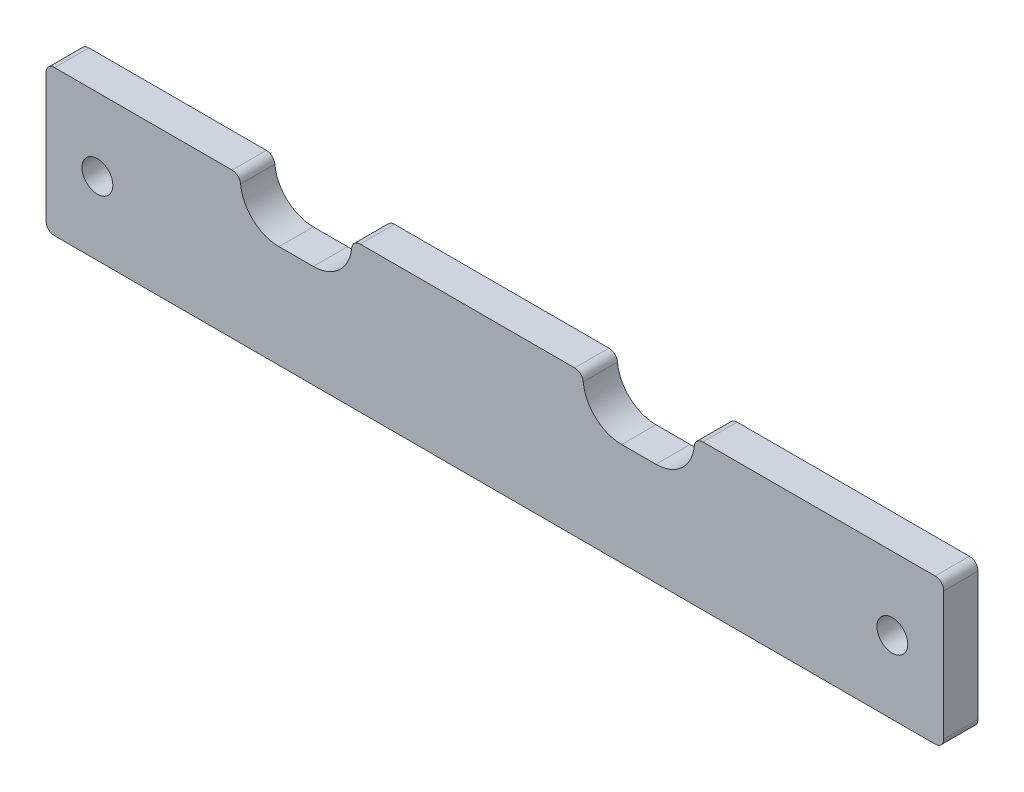
SolidWorks part; units mm, degrees
material "Q235B"
ref_plane "Front Plane" through (0, 0, 0) normal (0, 0, 1) x (1, 0, 0)
ref_plane "Top Plane" through (0, 0, 0) normal (0, 1, 0) x (1, 0, 0)
ref_plane "Right Plane" through (0, 0, 0) normal (1, 0, 0) x (0, 0, -1)
sketch "Sketch1" plane through (0, 0, 0) normal (0, 0, 1) x (1, 0, 0)
  line L0 (-26685.0454, 9467.9632) -> (-26685.0454, 9542.9632)
  line L1 (-26161.0454, 9467.9632) -> (-26161.0454, 9542.9632)
  line L2 (-26166.0454, 9462.9632) -> (-26680.0454, 9462.9632)
  line L3 (-26549.0454, 9522.9632) -> (-26529.0454, 9522.9632)
  line L4 (-26349.0454, 9522.9632) -> (-26329.0454, 9522.9632)
  line L5 (-26680.0454, 9547.9632) -> (-26576.4315, 9547.9632)
  line L6 (-26501.6593, 9547.9632) -> (-26376.4315, 9547.9632)
  line L7 (-26301.6593, 9547.9632) -> (-26289.0454, 9547.9632)
  line L8 (-26289.0454, 9547.9632) -> (-26166.0454, 9547.9632)
  circle A0 centre (-26655.0454, 9505.4632) radius 9
  circle A1 centre (-26191.0454, 9505.4632) radius 9
  arc A2 (-26571.4522, 9543.4178) -> (-26549.0454, 9522.9632) centre (-26549.0454, 9545.4632) ccw
  arc A3 (-26529.0454, 9522.9632) -> (-26506.6386, 9543.4178) centre (-26529.0454, 9545.4632) ccw
  arc A4 (-26371.4522, 9543.4178) -> (-26349.0454, 9522.9632) centre (-26349.0454, 9545.4632) ccw
  arc A5 (-26329.0454, 9522.9632) -> (-26306.6386, 9543.4178) centre (-26329.0454, 9545.4632) ccw
  arc A6 (-26571.4522, 9543.4178) -> (-26576.4315, 9547.9632) centre (-26576.4315, 9542.9632) ccw
  arc A7 (-26501.6593, 9547.9632) -> (-26506.6386, 9543.4178) centre (-26501.6593, 9542.9632) ccw
  arc A8 (-26371.4522, 9543.4178) -> (-26376.4315, 9547.9632) centre (-26376.4315, 9542.9632) ccw
  arc A9 (-26301.6593, 9547.9632) -> (-26306.6386, 9543.4178) centre (-26301.6593, 9542.9632) ccw
  arc A10 (-26680.0454, 9547.9632) -> (-26685.0454, 9542.9632) centre (-26680.0454, 9542.9632) ccw
  arc A11 (-26685.0454, 9467.9632) -> (-26680.0454, 9462.9632) centre (-26680.0454, 9467.9632) ccw
  arc A12 (-26166.0454, 9462.9632) -> (-26161.0454, 9467.9632) centre (-26166.0454, 9467.9632) ccw
  arc A13 (-26161.0454, 9542.9632) -> (-26166.0454, 9547.9632) centre (-26166.0454, 9542.9632) ccw
  dimension "D1" = 464
extrude "Boss-Extrude1" add sketch "Sketch1" along normal blind 20
